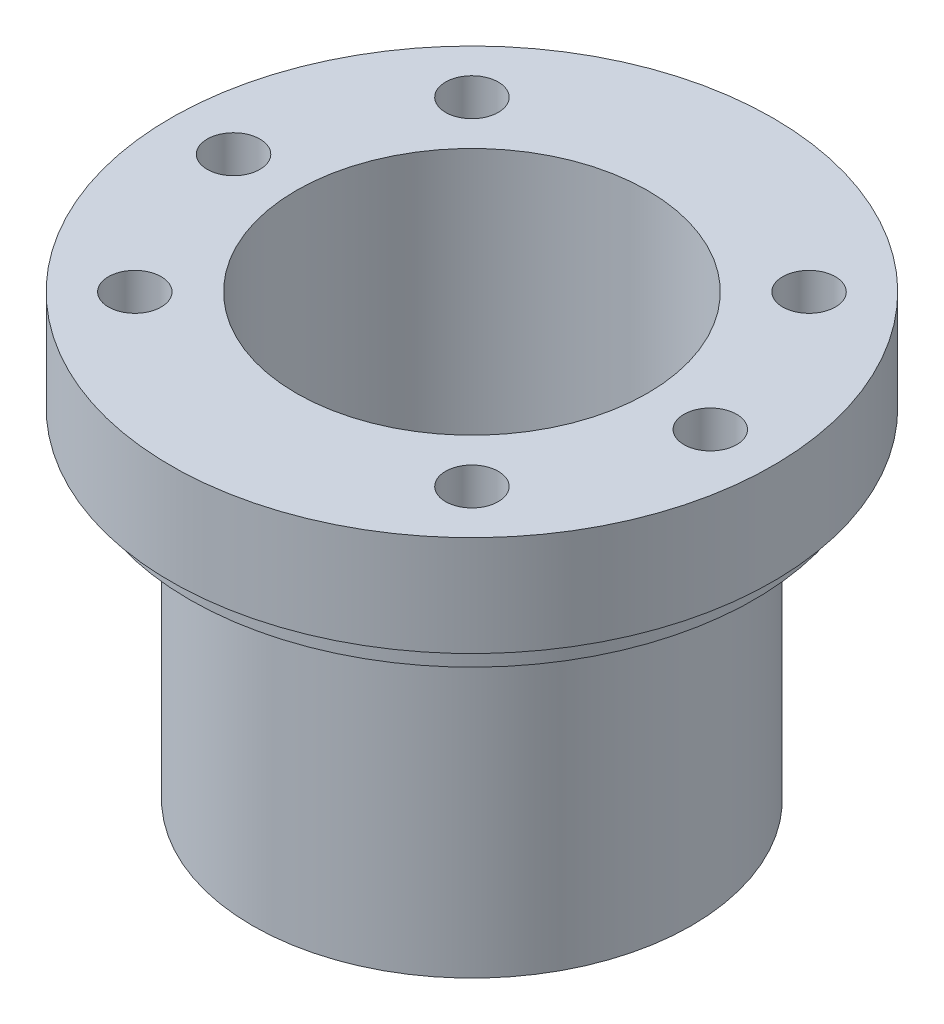
SolidWorks part; units mm, degrees
material "45"
ref_plane "Front Plane" through (0, 0, 0) normal (0, 0, 1) x (1, 0, 0)
ref_plane "Top Plane" through (0, 0, 0) normal (0, 1, 0) x (1, 0, 0)
ref_plane "Right Plane" through (0, 0, 0) normal (1, 0, 0) x (0, 0, -1)
sketch "Sketch1" plane through (0, 0, 0) normal (0, 0, 1) x (1, 0, 0)
  line L0 (14, 0) -> (17.5, 0)
  line L1 (17.5, 0) -> (17.5, 25)
  line L2 (17.5, 25) -> (22.5, 25)
  line L3 (24, 27) -> (24, 35)
  line L4 (24, 35) -> (14, 35)
  line L5 (14, 35) -> (14, 0)
  line L6 (0, 0) -> (0, 15.4104) construction
  line L7 (24, 27) -> (22.5, 27)
  line L8 (22.5, 27) -> (22.5, 25)
  dimension "D1" = 28
  dimension "D2" = 35
  dimension "D3" = 48
  dimension "D4" = 10
  dimension "D5" = 35
  dimension "D6" = 45
  dimension "D7" = 8
revolve "Revolve1" add sketch "Sketch1" angle 360 about L6
hole_wizard "M5 Tapped Hole1" positions "Sketch2" profile "Sketch3" tap size "M5" standard "GB"
sketch "Sketch2" plane through (0, 35, 0) normal (0, 1, 0) x (1, 0, 0)
  line L0 (19, 0) -> (0, 0)
  line L1 (0, 0) -> (-19, 0) construction
  line L3 (0, 0) -> (13.435, 13.435)
  line L6 (0, 0) -> (0, 17.3068) construction
  point P0 (-19, 0)
  point P2 (19, 0)
  point P14 (13.435, 13.435)
  point P28 (13.435, -13.435)
  point P30 (-13.435, -13.435)
  point P31 (-13.435, 13.435)
  dimension "D1" = 19
  dimension "D2" = 45
sketch "Sketch3" plane through (-19, 35, 0) normal (1, 0, 0) x (0, 0, 1)
  line L0 (0, 0) -> (0, 9.6618)
  line L1 (0, 9.6618) -> (2.1, 8.4)
  line L2 (2.1, 8.4) -> (2.1, 0)
  line L5 (2.1, 0) -> (0, 0)
  line L10 (0, 9.6618) -> (-2.1, 8.4) construction
  line L11 (0, -6.35) -> (0, 107.95) construction
  dimension "螺纹孔钻头直径" = 4.2
  dimension "螺纹孔钻头深度" = 8.4
  dimension "导头角度" = 118
cosmetic thread "Hole Thread1"
cosmetic thread "Hole Thread2"
cosmetic thread "Hole Thread3"
cosmetic thread "Hole Thread4"
cosmetic thread "Hole Thread5"
cosmetic thread "Hole Thread6"
